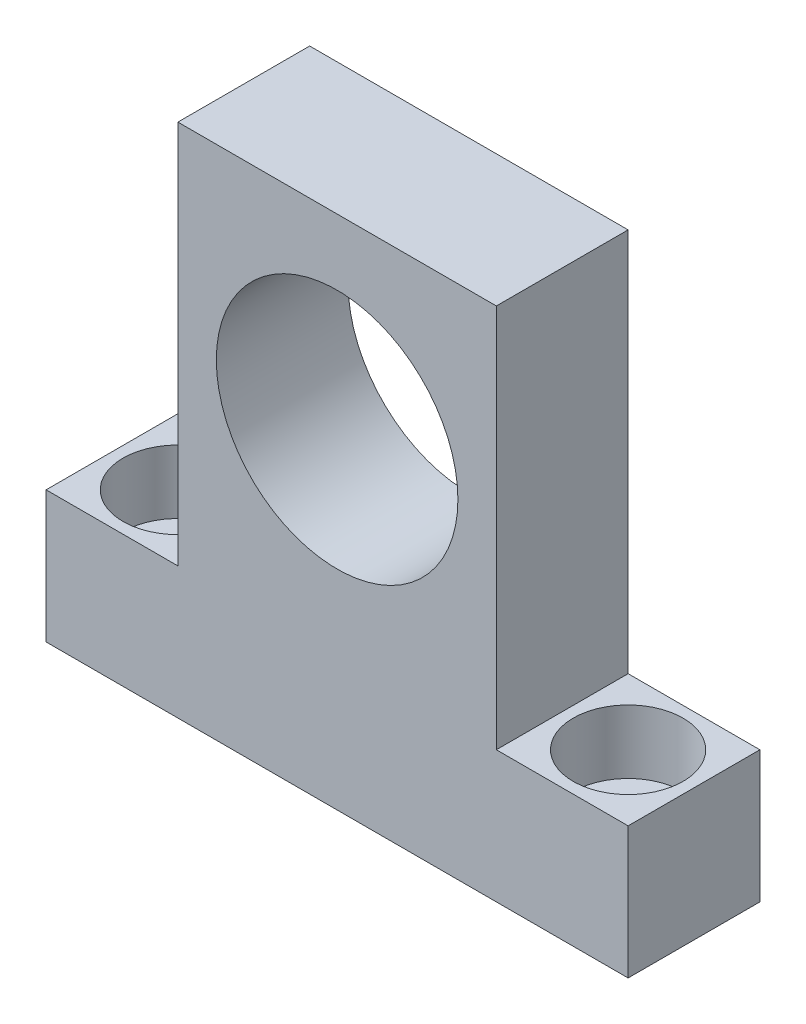
from build123d import *

# Parameters (mm, degrees)
SKETCH_1_R          = 11
EXTRUDE_1_DEPTH     = 12
SKETCH_2_R          = 2.75
CUT_EXTRUDE_1_DEPTH = 53.135542299
SKETCH_3_R          = 5
CUT_EXTRUDE_2_DEPTH = 5.8


with BuildPart() as part:
    # 草图1 → 凸台-拉伸1 (new body)
    with BuildSketch(Plane.XY):
        Polygon((-16.269702277, -16.03765324), (36.730297723, -16.03765324), (36.730297723, -4.03765324), (24.730297723, -4.03765324), (24.730297723, 30.96234676), (-4.269702277, 30.96234676), (-4.269702277, -4.03765324), (-16.269702277, -4.03765324), align=None)
        with Locations((10.230297723, 13.96234676)):
            Circle(SKETCH_1_R, mode=Mode.SUBTRACT)
    extrude(amount=EXTRUDE_1_DEPTH)

    # 草图2 → 切除-拉伸1 (cut, through all)
    with BuildSketch(Plane(origin=(0, -4.03765324, 0), x_dir=(1, 0, 0), z_dir=(0, 1, 0))):
        with Locations(Location((-10.269702277, -6, 0), (0, 0, 180))):
            Circle(SKETCH_2_R)
        with Locations(Location((30.730297723, -6, 0), (0, 0, 180))):
            Circle(SKETCH_2_R)
    extrude(amount=-CUT_EXTRUDE_1_DEPTH, mode=Mode.SUBTRACT)

    # 草图3 → 切除-拉伸2 (cut)
    with BuildSketch(Plane(origin=(0, -4.03765324, 0), x_dir=(1, 0, 0), z_dir=(0, 1, 0))):
        with Locations(Location((-10.269702277, -6, 0), (0, 0, 180))):
            Circle(SKETCH_3_R)
        with Locations(Location((30.730297723, -6, 0), (0, 0, 180))):
            Circle(SKETCH_3_R)
    extrude(amount=-CUT_EXTRUDE_2_DEPTH, mode=Mode.SUBTRACT)


solid = part.part
